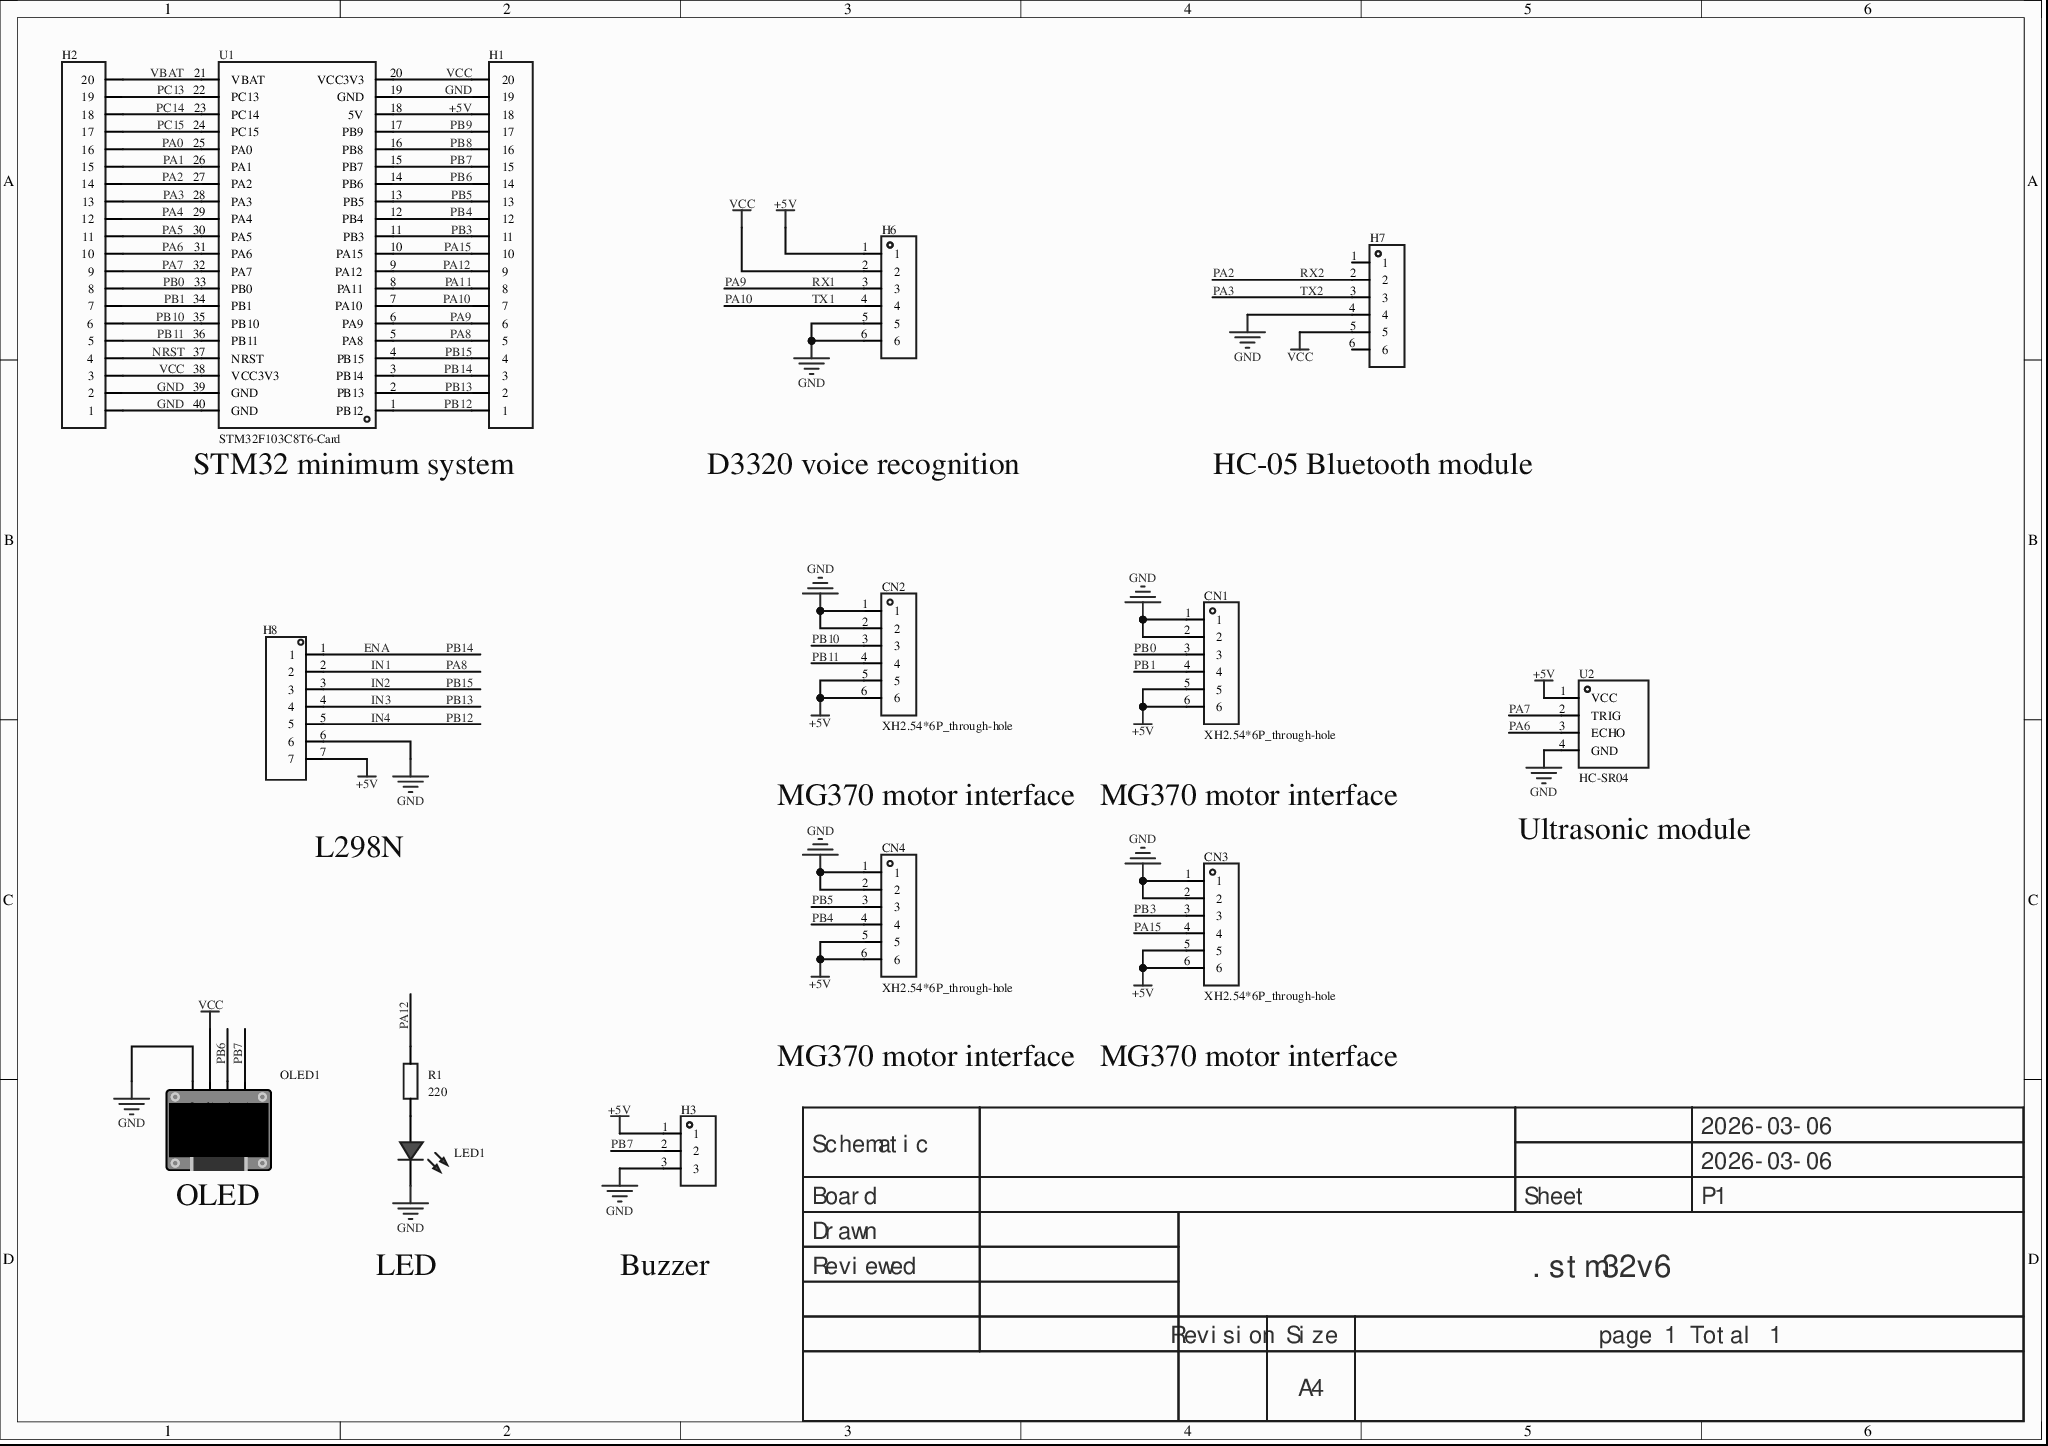
[diagram p0: MISC89099-3.schdoc]
# Altium project MISC89099-2.PrjPcb
1 sheet, 15 parts. Net scope: global (net labels, ports and power ports of the same name join across sheets).
Board file: MISC89099.pcbdoc

## Sheet MISC89099-3.schdoc
size 297 x 209 mm; Version: V1.0; @Project Name: MISC89099; @Page Count: 1; @Update Date: 2026-03-06; @Create Date: 2026-03-06; @Schematic Name: MISC89099; @Page No: 1; @Create Time: 23:22:16; @Update Time: 17:32:40; @Board Name: MISC89099

### Parts
CN1  XH2.54*6P_through-hole  [CONN-TH_XH2.54-6P]
CN2  XH2.54*6P_through-hole  [CONN-TH_XH2.54-6P]
CN3  XH2.54*6P_through-hole  [CONN-TH_XH2.54-6P]
CN4  XH2.54*6P_through-hole  [CONN-TH_XH2.54-6P]
H1  (no value)  [HDR-TH_20P-P2.54-V-F]
H2  (no value)  [HDR-TH_20P-P2.54-V-F]
H3  (no value)  [HDR-TH_3P-P2.54-V-F]
H6  (no value)  [HDR-TH_6P-P2.54-V-F]
H7  (no value)  [HDR-TH_6P-P2.54-V-F]
H8  (no value)  [HDR-TH_7P-P2.54-V-F]
LED1  (no value)  [LED_TH-3mm]
OLED1  (no value)  [0.96OLED_4P]
R1  220  [R0603]
U1  STM32F103C8T6-Card  [CONN-TH_L53.3-W22.9_STM32F103C8T6-CARD]
U2  HC-SR04  [TH_HC-SR04V]

### Nets
+5V: CN1.5 CN1.6 CN2.5 CN2.6 CN3.5 CN3.6 CN4.5 CN4.6 H1.18 H3.1 H6.1 H8.7 U1.18(5V) U2.1(VCC)
GND: CN1.1 CN1.2 CN2.1 CN2.2 CN3.1 CN3.2 CN4.1 CN4.2 H1.19 H2.1 H2.2 H3.3 H6.5 H6.6 H7.4 H8.6 LED1.2(A) OLED1.1(GND) U1.19(GND) U1.39(GND) U1.40(GND) U2.4(GND)
VCC: H1.20 H2.3 H6.2 H7.5 OLED1.2(VCC) U1.20(VCC3V3) U1.38(VCC3V3)
ENA: H1.3 H8.1 U1.3(PB14)  [also labelled PB14]
IN1: H1.5 H8.2 U1.5(PA8)  [also labelled PA8]
IN2: H1.4 H8.3 U1.4(PB15)  [also labelled PB15]
IN3: H1.2 H8.4 U1.2(PB13)  [also labelled PB13]
IN4: H1.1 H8.5 U1.1(PB12)  [also labelled PB12]
NRST: H2.4 U1.37(NRST)
PA0: H2.16 U1.25(PA0)
PA1: H2.15 U1.26(PA1)
PA2: H2.14 H7.2 U1.27(PA2)  [also labelled RX2]
PA3: H2.13 H7.3 U1.28(PA3)  [also labelled TX2]
PA4: H2.12 U1.29(PA4)
PA5: H2.11 U1.30(PA5)
PA6: H2.10 U1.31(PA6) U2.3(ECHO)
PA7: H2.9 U1.32(PA7) U2.2(TRIG)
PA9: H1.6 H6.3 U1.6(PA9)  [also labelled RX1]
PA10: H1.7 H6.4 U1.7(PA10)  [also labelled TX1]
PA11: H1.8 U1.8(PA11)
PA12: H1.9 R1.2 U1.9(PA12)
PA15: CN3.4 H1.10 U1.10(PA15)
PB0: CN1.3 H2.8 U1.33(PB0)
PB1: CN1.4 H2.7 U1.34(PB1)
PB3: CN3.3 H1.11 U1.11(PB3)
PB4: CN4.4 H1.12 U1.12(PB4)
PB5: CN4.3 H1.13 U1.13(PB5)
PB6: H1.14 OLED1.3(SCL) U1.14(PB6)
PB7: H1.15 H3.2 OLED1.4(SDA) U1.15(PB7)
PB8: H1.16 U1.16(PB8)
PB9: H1.17 U1.17(PB9)
PB10: CN2.3 H2.6 U1.35(PB10)
PB11: CN2.4 H2.5 U1.36(PB11)
PC13: H2.19 U1.22(PC13)
PC14: H2.18 U1.23(PC14)
PC15: H2.17 U1.24(PC15)
VBAT: H2.20 U1.21(VBAT)
NetLED1_1: LED1.1(C) R1.1

Not connected (* = marked no-connect by the designer): H7 1 6

### Notes on the sheet
- STM32 minimum system
- D3320 voice recognition
- HC-05 Bluetooth module
- L298N
- MG370 motor interface
- (near U2) Ultrasonic module
- OLED
- LED
- Buzzer
- 2026-03-06
- Schematic
- Board
- Sheet
- P1
- Drawn
- Reviewed
- .stm32v6
- Revision
- Size
- A4
- page 1 Total 1

### Library data of the parts
CN1-CN4 = XH2.54*6P_直插: AddInBom: yes; ModelId: a7224aacb0dc4305a7392217f7fd8fe20819f05c4eef4c71ace90d822a990e87; ModelTransform: 688.975,224.409,0,0,0,0,-0.001,-17.719,-118.11; Symbol: XH2.54*6P_through-hole; Device: XH2.54*6P_through-hole; LCSC Part Name: XH2.54*6P_直插; SupplierPart: C9900008614; ManufacturerPart: XH2.54*6P_直插; Supplier Footprint: XH2.54_6P; JLCPCB Part Class: Extended Part; Supplier: LCSC; ConvertToPcb: yes; FootprintName: CONN-TH_XH2.54-6P; ModelName: CONN-TH_XH2.54-6P
H1 H2 = HDR-F_2.54_1x20P: ConvertToPcb: yes; ModelId: db7015f7ad9d48b8a3b1188db02e3429; ModelName: HDR-F-2.54_1x20; ModelTransform: 1999.996,100,0,0,0,0,0,0,-118.11; Device: HDR-F_2.54_1x20P; Symbol: HDR-F_2.54_1x20P; AddInBom: yes; SupplierPart: C50984; Supplier Footprint: 插件; FootprintName: HDR-TH_20P-P2.54-V-F
H3 = HDR-F_2.54_1x3P: Symbol: PM254V-11-03-H85; 3D Model: f3b3cc5aae9641bf9e56fc160cef875b; 3D Model Transform: 299.9994,100,0,0,0,0,0,0,-118.11; ConvertToPcb: yes; ModelName: HDR2.54-F-LI-1X3P; Device: HDR-F_2.54_1x3P; Supplier Part: C541850; Supplier Footprint: 插件; AddInBom: yes; FootprintName: HDR-TH_3P-P2.54-V-F
H6 H7 = HDR-F_2.54_1x6P: Symbol: Header-Female-2.54_1x6; ConvertToPcb: yes; ModelId: 0f5bcf94dcda47d085f24cdca1696fe9; ModelTransform: 619.684,94.488,0,0,0,0,0,0,-125.984; Device: HDR-F_2.54_1x6P; AddInBom: yes; SupplierPart: C40877; Supplier Footprint: 插件; FootprintName: HDR-TH_6P-P2.54-V-F; ModelName: HDR-TH_6P-P2.54-V-F
H8 = HDR-F_2.54_1x7P: Symbol: 220S-1*7P H=8.5MM Ytype Gold-plated; ConvertToPcb: yes; ModelId: 4c31987253bc43b9b52c17be2a6d3f910819f05c4eef4c71ace90d822a990e87; ModelName: HDR-TH_7P-P2.54-F-LI-1X7P; ModelTransform: 715.7466,94.488,0,0,0,0,0,0,-118.11; Device: HDR-F_2.54_1x7P; AddInBom: yes; SupplierPart: C124418; Supplier Footprint: 插件; FootprintName: HDR-TH_7P-P2.54-V-F
LED1 = LED_TH-R_3mm: 3D Model: a497c992633541038a38947cdc58012f0819f05c4eef4c71ace90d822a990e87; 3D Model Transform: 141.274,153.327,0,0,0,0,-5.984,0,-137.795; ConvertToPcb: yes; ModelName: LED-TH-3mm_R; Symbol: LED_TH-R; Device: LED_TH-R_3mm; Supplier Footprint: 插件; AddInBom: yes; FootprintName: LED_TH-3mm
OLED1 = 0.96OLED模块_4P: Symbol: 0.96OLED module_4P; 3D Model: 79c000fdb68d45a296c2e9bedf4f9055; 3D Model Transform: 1393.69792,1318.895,0,0,0,0,0,-560.079,-137.795; ConvertToPcb: yes; Device: 0.96OLED module_4P; Supplier Footprint: 插件; AddInBom: yes; FootprintName: 0.96OLED_4P; ModelName: 0.96OLED_4P
R1 = Res_0603: Symbol: Resistor; 3D Model: fc143cca1e79419f9cd78b61e9279f080819f05c4eef4c71ace90d822a990e87; 3D Model Transform: 31.8897,63.7794,0,90,0,0,0,0,0; ConvertToPcb: yes; Device: Res_0603; Supplier Footprint: 0603; Value: 220; AddInBom: yes; FootprintName: R0603; ModelName: R0603
U1 = STM32F103C8T6-Card: AddInBom: yes; Symbol: STM32F103C8T6-CARD; Device: STM32F103C8T6-Card; LCSC Part Name: STM32F103C8T6-Card; SupplierPart: C9900077949; ManufacturerPart: STM32F103C8T6-Card; Supplier Footprint: 插件; Supplier: LCSC; ConvertToPcb: yes; FootprintName: CONN-TH_L53.3-W22.9_STM32F103C8T6-CARD
U2 = HC-SR04: Manufacturer: Universal Microelectronics; AddInBom: yes; Symbol: HC-SR04; Device: HC-SR04; LCSC Part Name: HC-SR04; SupplierPart: C19857336; ManufacturerPart: HC-SR04; Supplier Footprint: -; JLCPCB Part Class: Extended library; Datasheet: https://atta.szlcsc.com/upload/public/pdf/source/20240122/47B8E374E428935B7962A2189EF91AAC.pdf; Supplier: LCSC; ConvertToPcb: yes; FootprintName: TH_HC-SR04V